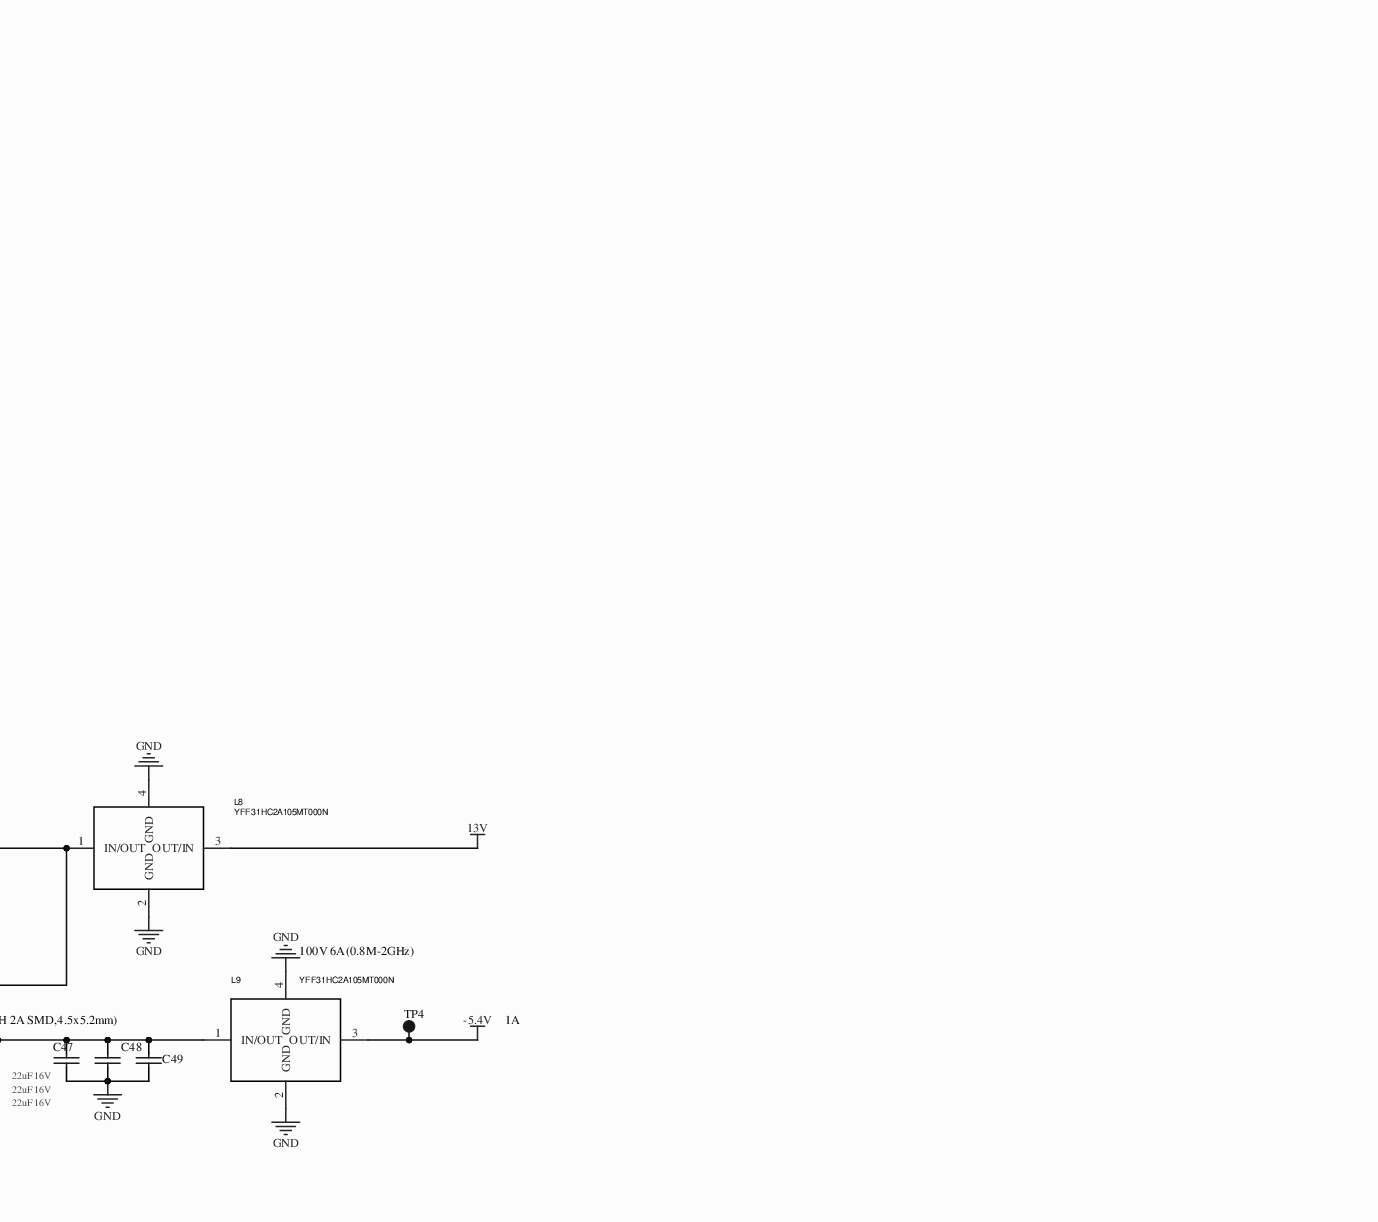
[diagram p0: MISC82191-5.SchDoc, bottom middle]
# Altium project MISC82191-2.PrjPcb (part 3 of 4)
## Sheet MISC82191-5.SchDoc (continued)
### Parts (continued)
C4  10uf  [0805A]
C5  22uF/16V  [0805]
C6  100nF  [0603]
C7  100nF  [0603]
C8  10uF 25V  [0805]
C9  4.7uF 25V  [0603]
C10  100nF 25V  [0603]
C11  100nF 25V  [0603]
C12  10nF  [0603]
C13  100nF  [0402]
C14  22uF/16V  [0805]
C15  220UF 25V (D6.3*7.7mm)  [CAP-SMD-6.3]
C16  100NF 10%  [0603]
C17  100nF 25V  [0603]
C18  47uF 25V  [1206]
C19  47uF 25V  [1206]
C20  10nF 25V  [0603]
C21  8200pF 25V  [0603]
C23  220UF 25V (D6.3*7.7mm)  [CAP-SMD-6.3]
C24  330nF 10%  [0805]
C25  100nF 10%  [0805]
C26  47uF 25V  [1206]
C27  47uF 25V  [1206]
C35  47uF 25V  [1206]
C36  47uF 25V  [1206]
C37  100nF 10%  [0805]
C38  220UF 25V (D6.3*7.7mm)  [CAP-SMD-6.3]
C39  330nF 10%  [0805]
C40  220nF 25V  [0603]
C41  2.2uF 25V  [0603]
C42  22uF 25V  [1206]
C43  22uF 25V  [1206]
C44  10uF 16V  [0603]
C45  10uF 16V  [0603]
C46  10uF 16V  [0603]
C47  22uF 16V  [0805]
C48  22uF 16V  [0805]
C49  22uF 16V  [0805]
C50  1uF 25V  [0603]
CN1  ZX-XH2.54-2PZZ  [CONN-TH_2P-P2.50_HX25003-2A]  (value not drawn)
D1  SB1045L  [SB1045L]
F2  16V 4A  [1812]
IC1  TPL910A  [DFN-8_L3.0-W3.0-P0.65-BL-EP2.3]
J100  DC-044A-A250  [DC-IN-TH_DC-044A-A250]
J300  WJ15EDGVC-3.81-2P  [CONN-TH_WJ15EDGVC-3.81-2P]
L1  YFF31HC2A105MT000N  [FILTER-SMD_4P-L3.2-W1.6-L_YFF31HC]
L2  SLF0705-2R2MTT (2.2uH 6A)  [IND-SMD_L7.8-W7.0-A]
L3  YFF31HC2A105MT000N  [FILTER-SMD_4P-L3.2-W1.6-L_YFF31HC]
L4  YFF15PC0G435MT000N  [FILTER-SMD_4P-L1.0-W0.5-L]
L5  YFF31HC2A105MT000N  [FILTER-SMD_4P-L3.2-W1.6-L_YFF31HC]
L8  YFF31HC2A105MT000N  [FILTER-SMD_4P-L3.2-W1.6-L_YFF31HC]
L9  YFF31HC2A105MT000N  [FILTER-SMD_4P-L3.2-W1.6-L_YFF31HC]
L10  XRCD54-4R7M(4.7uH 2A SMD,4.5x5.2mm)  [IND-SMD_L7.8-W7.0-A]
R1  10K 1%  [0603]
R2  35.7K 1%  [0603]
R3  31.3K 1%  [0603]
R4  56K 1%  [0603]
R5  8.06K 1%  [0603]
R6  0R1%  [0805]
R7  10K 1%  [0603]
R8  80.6K 1%  [0603]
R9  1.69K 1%  [0603]
R12  100K 1%  [0603]
R13  143K 1%  [0603]
R14  24K 1%  [0603]
TP1  (no value)  [TP1]
TP2  (no value)  [TP1]
TP4  (no value)  [TP1]
U2  AMS1117S-1.8  [SOT-89-3_L4.5-W2.5-P1.50-LS4.2-BR]
U3  TPS54620RGYR  [VQFN-14_L3.5-W3.5-P0.50-BL-EP_TPS54622RHLT]
U5  L7809CD2T-TR(ST)  [TO-263-2_L10.0-W9.1-P5.08-LS15.2-TL]
U6  L7806CD2T-TR(ST)  [TO-263-2_L10.0-W9.1-P5.08-LS15.2-TL]
U7  TPS63710DRRR  [TDFN-12_L3.0-W3.0-P0.50-BL-EP]

### Nets
3V3: C4.2 L4.3(OUT/IN) U2.3(VIN)
9V 1.5A: C25.2 C26.2 C27.2 C38.1 C39.2 U5.3(Output) U6.1(Input)
13V: D1.3 L1.1(IN/OUT) L5.1(IN/OUT) L8.3(OUT/IN) R6.1
-5.4V: L9.3(OUT/IN) TP4.1
A6V: C35.2 C36.2 C37.2 U6.3(Output)
D5V: C5.2 C6.2 IC1.5(EN) IC1.7(IN) IC1.8(IN) L3.3(OUT/IN) TP1.1
DGND: C3.2 C4.1 C5.1 C6.1 C7.1 C8.2 C9.2 C10.2 C13.1 C14.1 C15.2 C16.2 C17.2 C18.2 C19.2 C20.2 C21.2 C23.2 C24.1 C25.1 C26.1 C27.1 C35.1 C36.1 C37.1 C38.2 C39.1 C40.1 C41.2 C42.2 C43.2 C47.1 C48.1 C49.1 C50.2 CN1.2 IC1.4(GND) IC1.9(pad) J100.2 J100.3 J300.2 L1.2(GND) L1.4(GND) L3.2(GND) L3.4(GND) L4.2(GND) L4.4(GND) L5.2(GND) L5.4(GND) L8.2(GND) L8.4(GND) L9.2(GND) L9.4(GND) R1.1 R5.2 R7.2 R8.2 R14.2 U2.1(GND) U3.2(GND) U3.3(GND) U3.15(EP) U5.4(Ground) U6.4(Ground) U7.9(GND) U7.10(GND) U7.13(EP)  [also labelled GND]
VCC1V8: C3.1 U2.2(VOUT)
NetC7_2: C7.2 IC1.6(RN)
NetC8_1: C8.1 C9.1 C10.1 C15.1 C16.1 L1.3(OUT/IN) R2.1 U3.4(PVIN) U3.5(PVIN) U3.6(VIN)
NetC11_1: C11.1 U3.13(BOOT)
NetC11_2: C11.2 L2.2 U3.11(PH) U3.12(PH)
NetC12_1: C12.1 IC1.3(FB) R1.2 R3.1
NetC12_2: C12.2 C13.2 C14.2 IC1.1(OUT) IC1.2(OUT) L4.1(IN/OUT) R3.2 TP2.1
NetC17_1: C17.1 C18.1 C19.1 L2.1 L3.1(IN/OUT) R4.2
NetC20_1: C20.1 U3.9(SS/TR)
NetC21_1: C21.1 R9.2
NetC23_1: C23.1 C24.2 L5.3(OUT/IN) U5.1(Input)
NetC40_2: C40.2 U7.1(VAUX)
NetC41_1: C41.1 C42.1 C43.1 L8.1(IN/OUT) U7.2(EN) U7.12(VIN)
NetC44_1: C44.1 C45.1 C46.1 L10.2 U7.8(SW)
NetC44_2: C44.2 C45.2 C46.2 U7.11(CP)
NetC47_2: C47.2 C48.2 C49.2 L9.1(IN/OUT) L10.1 U7.7(VOUT)
NetC50_1: C50.1 U7.6(CAP)
NetCN1_1: CN1.1 R6.2
NetD1_1: D1.1 D1.2 F2.2
NetF2_1: F2.1 J100.1 J300.1
NetR2_2: R2.2 R5.1 U3.10(EN)
NetR4_1: R4.1 R7.1 U3.7(VSENSE)
NetR8_1: R8.1 U3.1(RT/CLK)
NetR9_1: R9.1 U3.8(COMP)
NetR12_2: R12.2 U7.3(PG)
NetR13_1: R13.1 R14.1 U7.5(FB)
NetR13_2: R13.2 U7.4(VREF)

Not connected (* = marked no-connect by the designer): J100 4 5; R12 1; U3 14(PWRGD)

### Notes on the sheet
- (near L1) 100V 6A(0.8M-2GHz)
- 13V@10A
- (near U3) 5V 6A
- (near L3) 100V 6A(0.8M-2GHz)
- (near D1) 0.5V@5A
- (near L4) 4V 2A (0.2M--1GHz)
- 3.3V 1A
- (near L9) 100V 6A(0.8M-2GHz)
- (near R13) When the output is 5.3V, change 143K to 140K
- 1A

### Library data of the parts
C3 = CAPACITOR: Generic Capacitor; DPN: *; Manufacturer: *; Value: 22uF
C4 = CAPACITOR: Generic Capacitor; Value: 22uF; DPN: *; Manufacturer: *
C5 C12-C14 = C1206
C6 C7 = C0402
C8-C11 C16-C21 C24-C27 C35-C37 C39-C50 = CAP: Capacitor
C15 C23 C38 = CAPACITOR_1: Capacitor
CN1 = ZX-XH2.54-2PZZ: Add into BOM: yes; Pins Structure: 1x2P; Pitch: 2.54mm; Reference Series: XH; Number of PINs Per Row: 2; Current Rating (Max): 3A; Symbol: ZX-XH2.54-2PZZ; Device: ZX-XH2.54-2PZZ; LCSC Part Name: ZX-XH2.54-2PZZ; Supplier Part: C7429632; Manufacturer Part: ZX-XH2.54-2PZZ; JLCPCB Part Class: Extended Part; Datasheet: https://atta.szlcsc.com/upload/public/pdf/source/20230619/19BA6947230AA44A04D3EDD65E618FD0.pdf; Supplier: LCSC; Convert to PCB: yes; Number of Pins: 2P; Number of Rows: 1; Row Spacing: -; Comment_1: ZX-XH2.54-2PZZ
F2 = Fuse 1: Fuse
IC1 = TPL910A: 3PEAK
J100 = DC-044A-A250: Manufacturer: XUNPU(讯普); Add into BOM: yes; Connector Type: DC power jack; Inside Contact Diameter: 2.5mm; Outside Contact Diameter: 5.9mm; Current Rating (Max): 3A; Voltage Rating (Max): 30V; Symbol: DC-044A-A250; Device: DC-044A-A250; LCSC Part Name: DC电源插座 内径:2.5mm 外径:5.9mm; Supplier Part: C720576; Manufacturer Part: DC-044A-A250; Supplier Footprint: 插件; JLCPCB Part Class: Extended Part; Datasheet: https://atta.szlcsc.com/upload/public/pdf/source/20240409/5208DBDD789FB06E905FC2EDCBF5D824.pdf; Supplier: LCSC; Convert to PCB: yes; Mounting Style: Right-angle; Operating Temperature Range: -20℃~+70℃
J300 = WJ15EDGVC-3.81-2P: Manufacturer: KANGNEX(康奈克斯电气); Add into BOM: yes; Connector Type: Board end/socket-closed; Structure: 1x2P; Pitch: 3.81mm; Number of PINs Per Row: 2; Current Rating (Max): 8A; Voltage Rating (Max): 300V; Symbol: WJ15EDGVC-3.81-2P; Device: WJ15EDGVC-3.81-2P; LCSC Part Name: 1x2P 3.81mm 排数:1 每排P数:2; Supplier Part: C8396; Manufacturer Part: WJ15EDGVC-3.81-2P; Supplier Footprint: 插件,P=3.81mm; JLCPCB Part Class: Extended Part; Datasheet: https://atta.szlcsc.com/upload/public/pdf/source/20191225/C8396_DFFE6D58C2AF45781C2AF0BF2B733CCC.pdf; Supplier: LCSC; Convert to PCB: yes; fixed form: -; Color: -; Mounting Style: Straight pin; Number of Pins: 2P; Number of Rows: 1; Wire Gauge - AWG: -; Wire Gauge - mm2: -; Contact Material: Brass; Contact Plating: Tin; Operating Temperature Range: -40℃~+105℃; Soldering Temperature(Max): -; Connection Type: -; Outlet Direction (Vertical Basis): -
L1 L3-L5 L8 L9 = YFF31HC2A105MT000N: as L104 on sheet MISC82191-3; Name: YFF31HC2A105MT000N; Symbol: YFF31HC2A105MT000N; Device: YFF31HC2A105MT000N; LCSC Part Name: 1uF(105) ±20% 100V; Supplier Part: C113216; Manufacturer Part: YFF31HC2A105MT000N; Supplier Footprint: SMD-4P,1.6x3.2mm; JLCPCB Part Class: Extended Part; Datasheet: https://atta.szlcsc.com/upload/public/pdf/source/20180326/C113216_F6F81E50B9805DA3D7C436129903DEBD.pdf; Supplier: LCSC; Convert to PCB: yes; Operating Temperature: -55℃~+125℃
L2 L10 = L
R1 R3 R6 = R0603: Value: NM
R2 R4 R5 R7-R9 R12-R14 = RES1
TP1 TP2 TP4 = TEST_2
U2 = AMS1117S-3.3
U3 = TPS54620RGYR: Manufacturer: TI(德州仪器); Add into BOM: yes; Function: Buck; Output Type: Adjustable; Input Voltage: 4.5V~17V; Output Voltage: 800mV~15V; Output Current (Max): 6A; Switching Frequency: 1.6MHz; Number of Outputs: 1; Switch tube (built-in/external): Built-in; Name: TPS54620RGYR; Symbol: TPS54620RGYR; Device: TPS54620RGYR; LCSC Part Name: TPS54620RGYR; Supplier Part: C29438; Manufacturer Part: TPS54620RGYR; Supplier Footprint: VQFN-14-EP(3.5x3.5); JLCPCB Part Class: Extended Part; Datasheet: https://www.ti.com/cn/lit/gpn/tps54620; Supplier: LCSC; Convert to PCB: yes; Operating Temperature: -40℃~+150℃@(TJ); Synchronous Rectification: Yes; Topology: Buck
U5 U6 = L7809CD2T-TR: Manufacturer: ST(意法半导体); Add into BOM: yes; Output Type: Fixed; Maximum Input Voltage: 35V; Output Voltage: 9V; MAX Output Current: 1.5A; Power Supply Rejection Ratio (PSRR): 55dB@(120Hz); Dropout Voltage: 2V@(1A); standby current: 8mA; Output Polarity: Positive; Number of Outputs: 1; Name: L7809CD2T-TR; Symbol: L7809CD2T; Device: L7809CD2T-TR; LCSC Part Name: 输入35V 输出9V 1.5A; Supplier Part: C20525; Manufacturer Part: L7809CD2T-TR; Supplier Footprint: TO-263-2; JLCPCB Part Class: Extended Part; Datasheet: https://atta.szlcsc.com/upload/public/pdf/source/20140724/1457707162800.pdf; Supplier: LCSC; Convert to PCB: yes; Operating Temperature: 0℃~+125℃
U7 = TPS63710DRRR: Manufacturer: TI(德州仪器); Add into BOM: yes; Name: TPS63710DRRR; Symbol: TPS63710DRRR; Device: TPS63710DRRR; LCSC Part Name: TPS63710DRRR; Supplier Part: C485552; Manufacturer Part: TPS63710DRRR; Supplier Footprint: TDFN-12-EP(3x3); JLCPCB Part Class: Extended Part; Datasheet: https://www.ti.com/cn/lit/gpn/tps63710; Supplier: LCSC; Convert to PCB: yes